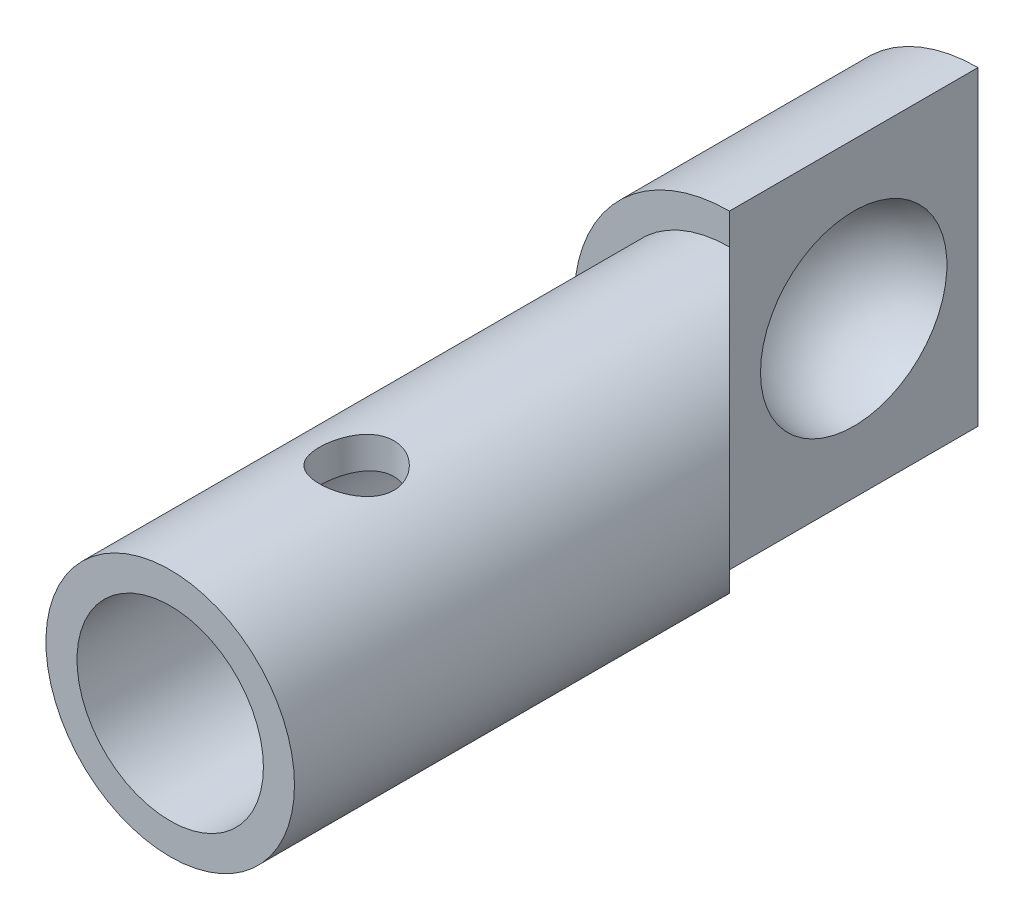
SolidWorks part; units mm, degrees
ref_plane "Front Plane" through (0, 0, 0) normal (0, 0, 1) x (1, 0, 0)
ref_plane "Top Plane" through (0, 0, 0) normal (0, 1, 0) x (1, 0, 0)
ref_plane "Right Plane" through (0, 0, 0) normal (1, 0, 0) x (0, 0, -1)
sketch "Sketch1" plane through (0, 0, 0) normal (0, 0, 1) x (1, 0, 0)
  circle A0 centre (0, 0) radius 7.5
  circle A1 centre (0, 0) radius 10
  dimension "D1" = 15
  dimension "D2" = 20
extrude "Boss-Extrude1" add sketch "Sketch1" along normal blind 45
sketch "Sketch2" plane through (0, 0, 0) normal (0, 1, 0) x (1, 0, 0)
  line L0 (-10, -45) -> (10, -45) construction
  circle A0 centre (0, -30) radius 3
  dimension "D1" = 6
  dimension "D2" = 15
extrude "Cut-Extrude1" cut sketch "Sketch2" against normal through all both and the other way through all
sketch "Sketch3" plane through (0, 0, 0) normal (0, 0, -1) x (-1, 0, 0)
  circle A0 centre (0, 0) radius 12.5
  dimension "D1" = 25
extrude "Boss-Extrude2" add sketch "Sketch3" along normal blind 20
sketch "Sketch4" plane through (0, 0, 0) normal (0, 1, 0) x (1, 0, 0)
  line L0 (12.5, 20) -> (-12.5, 20) construction
  line L1 (0, 20) -> (12.5, 20)
  line L2 (0, 20) -> (0, 0)
  line L4 (12.5, 20) -> (12.5, 0)
  line L5 (0, 0) -> (10, -10)
  line L6 (10, -45) -> (10, 0) construction
  line L7 (10, -10) -> (12.5, 0)
extrude "Cut-Extrude2" cut sketch "Sketch4" against normal through all both and the other way through all
sketch "Sketch5" plane through (0, 0, 0) normal (0, 1, 0) x (1, 0, 0)
  line L0 (0, 20) -> (0, 0) construction
  line L1 (0, 0) -> (0, 17.5) construction
  line L2 (0, 17.5) -> (0, 2.5)
  arc A0 (0, 17.5) -> (0, 2.5) centre (0, 10) ccw
  dimension "D1" = 15
revolve "Cut-Revolve3" cut sketch "Sketch5" angle 360 about L1
